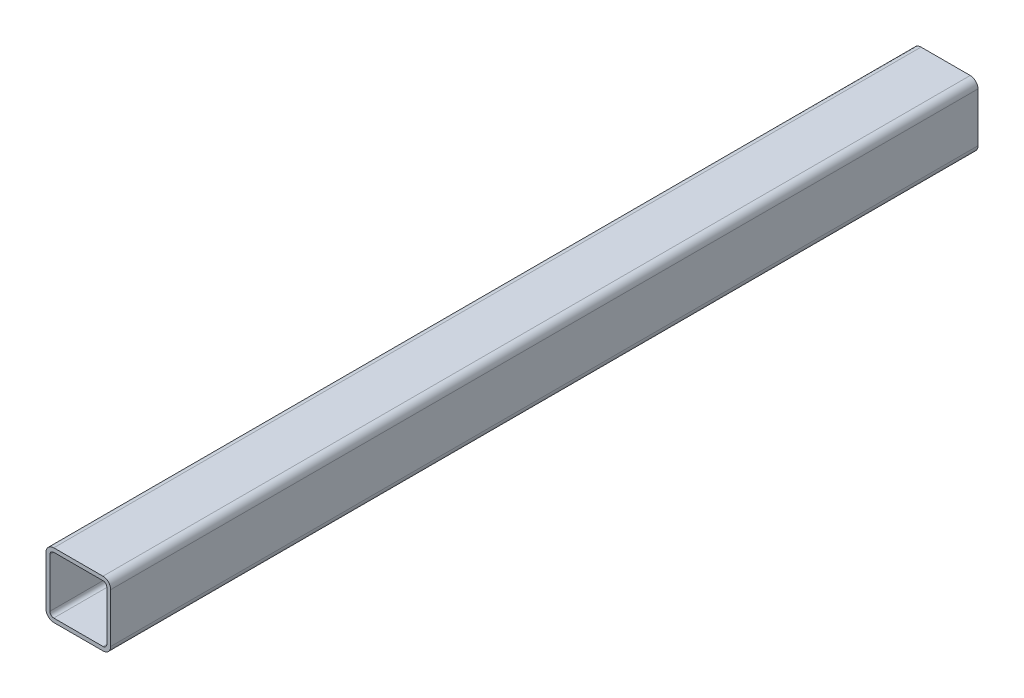
from build123d import *

# Parameters (mm, degrees)
GB_6728_1986_050_X_50_X_3_1_DEPTH = 670


with BuildPart() as part:
    # Sketch1 → Gb／6728-1986方形空心型钢 050 X 50 X 3(1) (new body)
    with BuildSketch(Plane.YX.offset(-335)):
        with BuildLine():
            Line((-19, -25), (19, -25))
            ThreePointArc((19, -25), (23.242640687, -23.242640687), (25, -19))
            Line((25, -19), (25, 19))
            ThreePointArc((25, 19), (23.242640687, 23.242640687), (19, 25))
            Line((19, 25), (-19, 25))
            ThreePointArc((-19, 25), (-23.242640687, 23.242640687), (-25, 19))
            Line((-25, 19), (-25, -19))
            ThreePointArc((-25, -19), (-23.242640687, -23.242640687), (-19, -25))
        make_face()
        with BuildLine():
            Line((-19, -22), (19, -22))
            ThreePointArc((19, -22), (21.121320344, -21.121320344), (22, -19))
            Line((22, -19), (22, 19))
            ThreePointArc((22, 19), (21.121320344, 21.121320344), (19, 22))
            Line((19, 22), (-19, 22))
            ThreePointArc((-19, 22), (-21.121320344, 21.121320344), (-22, 19))
            Line((-22, 19), (-22, -19))
            ThreePointArc((-22, -19), (-21.121320344, -21.121320344), (-19, -22))
        make_face(mode=Mode.SUBTRACT)
    extrude(amount=GB_6728_1986_050_X_50_X_3_1_DEPTH)


solid = part.part
